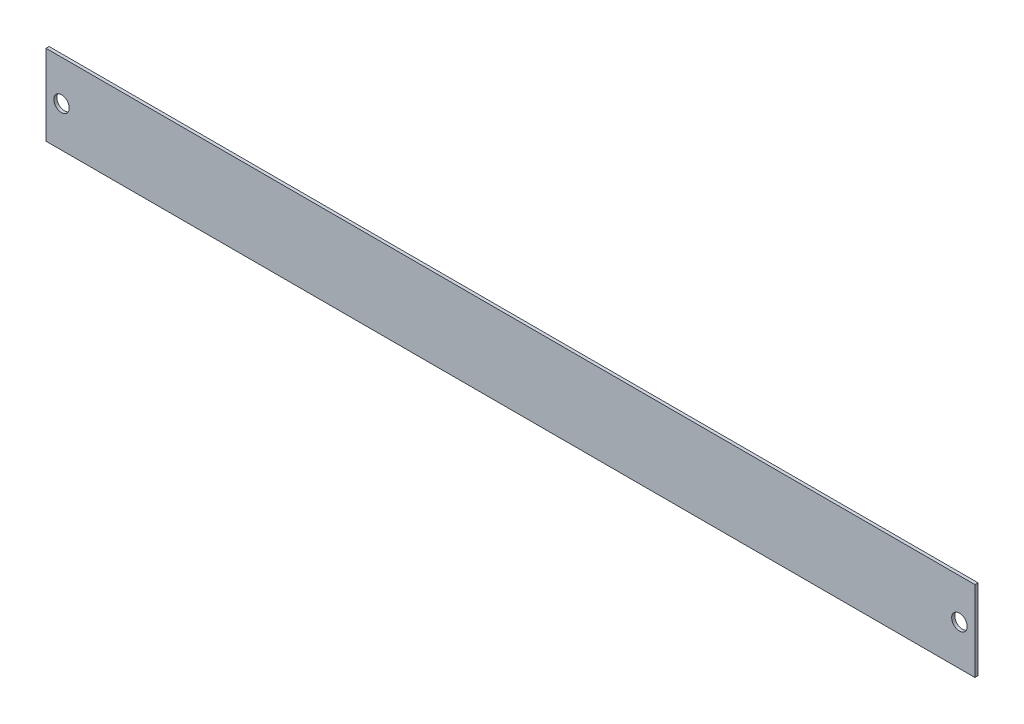
SolidWorks part; units mm, degrees
ref_plane "前视基准面" through (0, 0, 0) normal (0, 0, 1) x (1, 0, 0)
ref_plane "上视基准面" through (0, 0, 0) normal (0, 1, 0) x (1, 0, 0)
ref_plane "右视基准面" through (0, 0, 0) normal (1, 0, 0) x (0, 0, -1)
sketch "草图1" plane through (0, 0, 0) normal (0, 0, 1) x (1, 0, 0)
  line L1 (-150, 26) -> (150, 26)
  line L2 (-150, 26) -> (-150, 0)
  line L3 (-150, 0) -> (150, 0)
  line L4 (150, 26) -> (150, 0)
  dimension "D1" = 300
  dimension "D2" = 26
extrude "凸台-拉伸1" add sketch "草图1" along normal blind 1
hole_wizard "Ø5.0 (5) 直径孔1" positions "草图3" profile "草图2" hole size "Ø5.0" standard "GB"
sketch "草图3" plane through (0, 0, 1) normal (0, 0, 1) x (1, 0, 0)
  line L0 (-150, 26) -> (-150, 0) construction
  line L1 (-150, 13) -> (150, 13) construction
  line L2 (150, 0) -> (150, 26) construction
  point P0 (-145, 13)
  point P3 (145, 13)
  dimension "D1" = 5
  dimension "D2" = 5
sketch "草图2" plane through (-145, 13, 1) normal (1, 0, 0) x (0, -1, 0)
  line L0 (0, 0) -> (0, 6.5022)
  line L1 (0, 6.5022) -> (2.5, 5)
  line L2 (2.5, 5) -> (2.5, 0)
  line L5 (2.5, 0) -> (0, 0)
  line L10 (0, 6.5022) -> (-2.5, 5) construction
  line L11 (0, -6.35) -> (0, 107.95) construction
  dimension "孔直径" = 5
  dimension "孔深度" = 5
  dimension "导头角度" = 118
